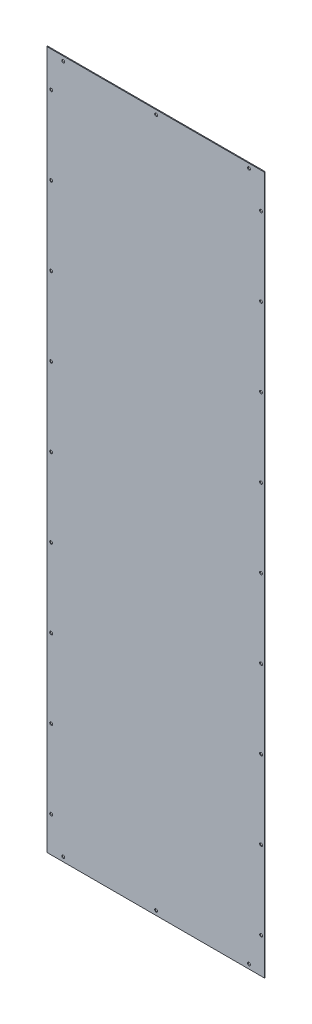
SolidWorks part; units mm, degrees
material "304"
ref_plane "前视基准面" through (0, 0, 0) normal (0, 0, 1) x (1, 0, 0)
ref_plane "上视基准面" through (0, 0, 0) normal (0, 1, 0) x (1, 0, 0)
ref_plane "右视基准面" through (0, 0, 0) normal (1, 0, 0) x (0, 0, -1)
sketch "草图1" plane through (0, 0, 0) normal (0, 0, 1) x (1, 0, 0)
  line L0 (0, 0) -> (451.2544, 0) construction
  line L1 (-247.25, 789) -> (247.25, 789)
  line L2 (-247.25, 789) -> (-247.25, -789)
  line L3 (-247.25, -789) -> (247.25, -789)
  line L4 (247.25, 789) -> (247.25, -789)
  line L5 (-247.25, 789) -> (247.25, -789) construction
  line L6 (-247.25, -789) -> (247.25, 789) construction
  line L7 (0, 0) -> (0, 412.8629) construction
  circle A0 centre (-237.25, 0) radius 3.25
  circle A1 centre (-237.25, -177.25) radius 3.25
  circle A2 centre (-237.25, -354.5) radius 3.25
  circle A3 centre (-237.25, -531.75) radius 3.25
  circle A4 centre (-237.25, -709) radius 3.25
  circle A34 centre (0, -779) radius 3.25
  circle A35 centre (0, 779) radius 3.25
  circle A36 centre (-237.25, 709) radius 3.25
  circle A37 centre (-237.25, 531.75) radius 3.25
  circle A38 centre (-237.25, 354.5) radius 3.25
  circle A39 centre (-237.25, 177.25) radius 3.25
  circle A40 centre (237.25, 177.25) radius 3.25
  circle A41 centre (237.25, 354.5) radius 3.25
  circle A42 centre (237.25, 531.75) radius 3.25
  circle A43 centre (237.25, 709) radius 3.25
  circle A44 centre (237.25, -709) radius 3.25
  circle A45 centre (237.25, -531.75) radius 3.25
  circle A46 centre (237.25, -354.5) radius 3.25
  circle A47 centre (237.25, -177.25) radius 3.25
  circle A48 centre (237.25, 0) radius 3.25
  circle A49 centre (-210, 779) radius 3.25
  circle A50 centre (210, 779) radius 3.25
  circle A51 centre (210, -779) radius 3.25
  circle A52 centre (-210, -779) radius 3.25
  point P0 (0, 0)
  point P49 (0, 0)
  point P50 (0, 0)
  dimension "D3" = 6.5
  dimension "D8" = 420
  dimension "D1" = 494.5
  dimension "D2" = 1578
  dimension "D4" = 10
  dimension "D6" = 10
  dimension "D7" = 80
  dimension "D5" = 5
extrude "凸台-拉伸1" add sketch "草图1" along normal blind 2
sketch "草图2" plane through (0, -789, 0) normal (0, -1, 0) x (1, 0, 0)
  line L0 (-247.25, 2) -> (247.25, 2) construction
  line L1 (247.25, 0) -> (244.75, 0)
  line L2 (247.25, 0) -> (247.25, 2)
  line L3 (247.25, 2) -> (244.75, 2)
  line L4 (244.75, 0) -> (244.75, 2)
  dimension "D1" = 2.5
extrude "切除-拉伸1" cut sketch "草图2" against normal through all
